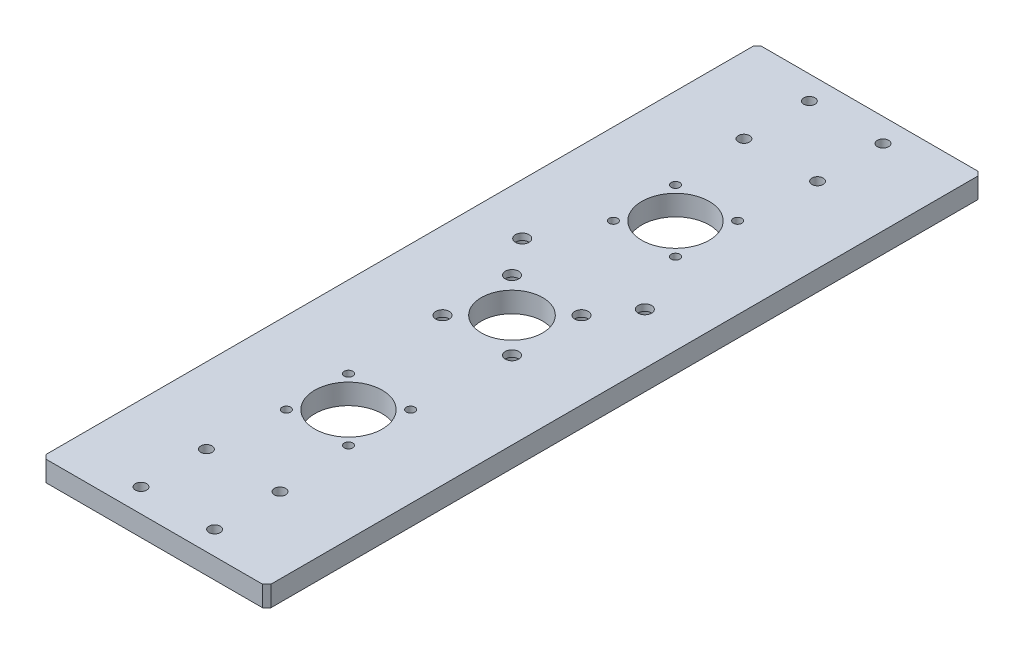
SolidWorks part; units mm, degrees
material "6061 Alloy"
ref_plane "Front Plane" through (0, 0, 0) normal (0, 0, 1) x (1, 0, 0)
ref_plane "Top Plane" through (0, 0, 0) normal (0, 1, 0) x (1, 0, 0)
ref_plane "Right Plane" through (0, 0, 0) normal (1, 0, 0) x (0, 0, -1)
sketch "Sketch1" plane through (0, 0, 0) normal (0, 1, 0) x (1, 0, 0)
  line L1 (-55, -175) -> (55, -175)
  line L2 (-55, -175) -> (-55, 175)
  line L3 (-55, 175) -> (55, 175)
  line L4 (55, -175) -> (55, 175)
  line L5 (-55, -175) -> (55, 175) construction
  line L6 (-55, 175) -> (55, -175) construction
  point P0 (0, 0)
  dimension "D1" = 350
  dimension "D2" = 110
extrude "Boss-Extrude1" add sketch "Sketch1" along normal blind 10
hole_wizard "Hole Size (% by) Socket Head Cap Screw Type1" positions "Sketch2" profile "Sketch3" counterbore size "M5" standard "GB" end condition up to next
sketch "Sketch2" plane through (0, 0, 0) normal (0, 1, 0) x (1, 0, 0)
  line L0 (-18, -131.5) -> (18, -131.5) construction
  line L1 (18, -131.5) -> (18, -163.5) construction
  line L2 (18, -163.5) -> (-18, -163.5) construction
  line L3 (-18, -163.5) -> (-18, -131.5) construction
  line L4 (0, -131.5) -> (0, 0) construction
  line L6 (0, 0) -> (55, 0) construction
  line L7 (55, -175) -> (55, 175) construction
  line L9 (-18, 163.5) -> (-18, 131.5) construction
  line L10 (18, 163.5) -> (-18, 163.5) construction
  line L11 (18, 131.5) -> (18, 163.5) construction
  line L12 (-18, 131.5) -> (18, 131.5) construction
  point P0 (-18, -131.5)
  point P2 (18, -131.5)
  point P7 (18, -163.5)
  point P9 (-18, -163.5)
  point P30 (18, -147.5)
  point P31 (-18, 163.5)
  point P32 (-18, 131.5)
  point P33 (18, 163.5)
  point P34 (18, 131.5)
  dimension "D1" = 32
  dimension "D2" = 36
  dimension "D3" = 295
sketch "Sketch3" plane through (-18, 0, 131.5) normal (1, 0, 0) x (0, 0, -1)
  line L0 (0, 0) -> (0, 10)
  line L1 (0, 10) -> (2.75, 10)
  line L3 (2.75, 10) -> (2.75, 5.7)
  line L4 (2.75, 5.7) -> (5, 5.7)
  line L5 (5, 5.7) -> (5, 0)
  line L7 (5, 0) -> (0, 0)
  line L11 (0, -6.35) -> (0, 107.95) construction
  dimension "通孔孔直径" = 5.5
  dimension "通孔孔深度" = 10
  dimension "柱形沉头孔直径" = 10
  dimension "柱形沉头孔深度" = 5.7
hole_wizard "Hole Size (% by) Socket Head Cap Screw Type2" positions "Sketch4" profile "Sketch5" counterbore size "M6" standard "GB" end condition up to next
sketch "Sketch4" plane through (0, 0, 0) normal (0, 1, 0) x (1, 0, 0)
  line L1 (-17, 17) -> (17, 17) construction
  line L2 (-17, 17) -> (-17, -17) construction
  line L3 (-17, -17) -> (17, -17) construction
  line L4 (17, 17) -> (17, -17) construction
  line L5 (-17, 0) -> (0, 0) construction
  line L6 (0, 0) -> (0, 17) construction
  point P0 (-17, 17)
  point P2 (17, 17)
  point P6 (17, -17)
  point P69 (-17, -17)
  dimension "D1" = 34
sketch "Sketch5" plane through (-17, 0, -17) normal (1, 0, 0) x (0, 0, -1)
  line L0 (0, 0) -> (0, 10)
  line L1 (0, 10) -> (3.3, 10)
  line L3 (3.3, 10) -> (3.3, 6.8)
  line L4 (3.3, 6.8) -> (5.5, 6.8)
  line L5 (5.5, 6.8) -> (5.5, 0)
  line L7 (5.5, 0) -> (0, 0)
  line L11 (0, -6.35) -> (0, 107.95) construction
  dimension "通孔孔直径" = 6.6
  dimension "通孔孔深度" = 10
  dimension "柱形沉头孔直径" = 11
  dimension "柱形沉头孔深度" = 6.8
chamfer "Chamfer1" distance 2 angle 45 4 edges at (-55, 5, -175) (55, 5, -175) (55, 5, 175) (-55, 5, 175)
hole_wizard "Hole Size (% by) Socket Head Cap Screw Type3" positions "Sketch6" profile "Sketch7" counterbore size "M6" standard "GB" end condition through all
sketch "Sketch6" plane through (0, 0, 0) normal (0, -1, 0) x (-1, 0, 0)
  line L0 (30, 35) -> (-30, 35) construction
  line L2 (0, 0) -> (0, 35) construction
  line L4 (-53, 175) -> (53, 175) construction
  point P0 (30, 35)
  point P2 (-30, 35)
  dimension "D1" = 60
  dimension "D2" = 140
sketch "Sketch7" plane through (-30, 0, -35) normal (1, 0, 0) x (0, 0, -1)
  line L0 (0, 0) -> (0, 10)
  line L1 (0, 10) -> (3.3, 10)
  line L3 (3.3, 10) -> (3.3, 6.8)
  line L4 (3.3, 6.8) -> (5.5, 6.8)
  line L5 (5.5, 6.8) -> (5.5, 0)
  line L7 (5.5, 0) -> (0, 0)
  line L11 (0, -6.35) -> (0, 107.95) construction
  dimension "通孔孔直径" = 6.6
  dimension "通孔孔深度" = 10
  dimension "柱形沉头孔直径" = 11
  dimension "柱形沉头孔深度" = 6.8
sketch "Sketch8" plane through (0, 0, 0) normal (0, -1, 0) x (1, 0, 0)
  line L0 (0, 0) -> (-109.894, 0) construction
  line L1 (0, -80) -> (0, 0) construction
  circle A0 centre (0, -80) radius 16.5
  circle A1 centre (0, 80) radius 16.5
  dimension "D1" = 33
  dimension "D2" = 160
extrude "Cut-Extrude1" cut sketch "Sketch8" against normal through all
hole_wizard "M5 Tapped Hole1" positions "Sketch9" profile "Sketch10" tap size "M5" standard "GB" end condition through all
sketch "Sketch9" plane through (0, 10, 0) normal (0, 1, 0) x (1, 0, 0)
  line L1 (-15.2028, 95.2028) -> (15.2028, 95.2028) construction
  line L2 (-15.2028, 95.2028) -> (-15.2028, 64.7972) construction
  line L3 (-15.2028, 64.7972) -> (15.2028, 64.7972) construction
  line L4 (15.2028, 95.2028) -> (15.2028, 64.7972) construction
  line L5 (-15.2028, 80) -> (0, 80) construction
  line L6 (0, 80) -> (0, 64.7972) construction
  line L7 (0, -80) -> (0, -95.2028) construction
  line L8 (-15.2028, -64.7972) -> (-15.2028, -95.2028) construction
  line L9 (-15.2028, -95.2028) -> (15.2028, -95.2028) construction
  line L10 (-15.2028, -80) -> (0, -80) construction
  line L11 (15.2028, -64.7972) -> (15.2028, -95.2028) construction
  line L12 (-15.2028, -64.7972) -> (15.2028, -64.7972) construction
  circle A0 centre (0, 80) radius 21.5 construction
  circle A1 centre (0, -80) radius 21.5 construction
  point P0 (-15.2028, 95.2028)
  point P4 (15.2028, 64.7972)
  point P8 (15.2028, 64.7972)
  point P87 (-15.2028, 64.7972)
  point P88 (15.2028, 95.2028)
  point P110 (-15.2028, -64.7972)
  point P111 (15.2028, -95.2028)
  point P124 (-15.2028, -64.7972)
  point P127 (15.2028, -64.7972)
  point P130 (15.2028, -95.2028)
  point P133 (-15.2028, -95.2028)
  dimension "D1" = 43
  dimension "D2" = 43
sketch "Sketch10" plane through (-15.2028, 10, -95.2028) normal (1, 0, 0) x (0, 0, 1)
  line L0 (0, 0) -> (0, 10)
  line L1 (0, 10) -> (2.1, 10)
  line L2 (2.1, 10) -> (2.1, 0)
  line L5 (2.1, 0) -> (0, 0)
  line L11 (0, -6.35) -> (0, 107.95) construction
  dimension "通孔螺纹孔钻头直径" = 4.2
  dimension "通孔螺纹孔钻头深度" = 10
cosmetic thread "Hole Cosmetic Thread1" parameters "D2"=5
cosmetic thread "Hole Cosmetic Thread2" parameters "D2"=5
cosmetic thread "Hole Cosmetic Thread3" parameters "D2"=5
cosmetic thread "Hole Cosmetic Thread4" parameters "D2"=5
cosmetic thread "Hole Cosmetic Thread6" parameters "D2"=5
cosmetic thread "Hole Cosmetic Thread7" parameters "D2"=5
cosmetic thread "Hole Cosmetic Thread8" parameters "D2"=5
cosmetic thread "Hole Cosmetic Thread9" parameters "D2"=5
cosmetic thread "Hole Cosmetic Thread10" parameters "D2"=5
cosmetic thread "Hole Cosmetic Thread11" parameters "D2"=5
cosmetic thread "Hole Cosmetic Thread12" parameters "D2"=5
sketch "Sketch11" plane through (0, 10, 0) normal (0, 1, 0) x (1, 0, 0)
  circle A0 centre (0, 0) radius 15
  dimension "D1" = 30
extrude "Cut-Extrude2" cut sketch "Sketch11" against normal through all
